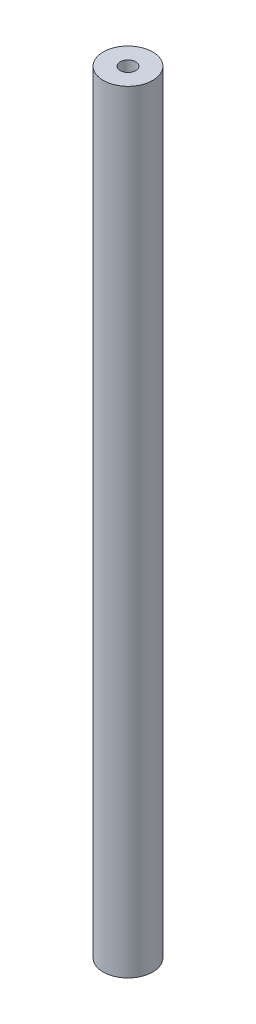
from build123d import *

# Parameters (mm, degrees)
SKETCH_1_R             = 8
EXTRUDE_1_DEPTH        = 250
HOLE_WIZARD_M6_1_D     = 5
HOLE_WIZARD_M6_1_DEPTH = 15
HOLE_WIZARD_M6_1_TIP   = 1.502151548


with BuildPart() as part:
    # 草图1 → 凸台-拉伸1 (new body)
    with BuildSketch(Plane(origin=(0, 0, 0), x_dir=(1, 0, 0), z_dir=(0, 1, 0))):
        with Locations(Location((0, 0, 0), (0, 0, 270))):
            Circle(SKETCH_1_R)
    extrude(amount=EXTRUDE_1_DEPTH)

    # M6 螺纹孔1
    with Locations(Plane(origin=(0, 250, 0), x_dir=(1, 0, 0), z_dir=(0, 1, 0))):
        with Locations((0, 0)):
            Hole(HOLE_WIZARD_M6_1_D / 2, depth=HOLE_WIZARD_M6_1_DEPTH)
            with Locations((0, 0, -(HOLE_WIZARD_M6_1_DEPTH + HOLE_WIZARD_M6_1_TIP / 2))):  # 118° drill point
                Cone(0, HOLE_WIZARD_M6_1_D / 2, HOLE_WIZARD_M6_1_TIP, mode=Mode.SUBTRACT)


solid = part.part
